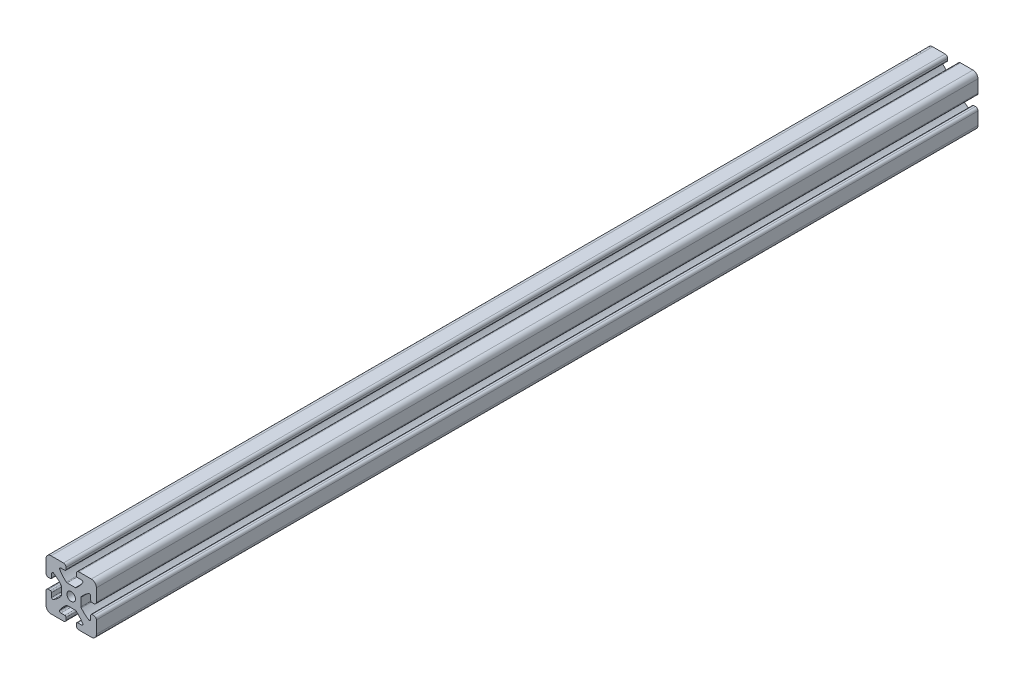
from build123d import *

# Parameters (mm, degrees)
SKETCH1_R           = 3.4
BOSS_EXTRUDE1_DEPTH = 700


with BuildPart() as part:
    # Sketch1 → Boss-Extrude1 (new body)
    with BuildSketch(Plane.XY):
        with BuildLine():
            Line((-72.552625451, -20.1458069), (-75.708839475, -20.1458069))
            ThreePointArc((-75.708839475, -20.1458069), (-76.585125865, -19.62759748), (-76.55321253, -18.610051226))
            ThreePointArc((-76.55321253, -18.610051226), (-74.186362214, -15.403020453), (-71.332517782, -12.620467892))
            ThreePointArc((-71.332517782, -12.620467892), (-71.036129936, -12.453644757), (-70.700972516, -12.3958069))
            Line((-70.700972516, -12.3958069), (-67.452625451, -12.3958069))
            Line((-67.452625451, -12.3958069), (-64.204278386, -12.3958069))
            ThreePointArc((-64.204278386, -12.3958069), (-63.869120967, -12.453644757), (-63.572733121, -12.620467892))
            ThreePointArc((-63.572733121, -12.620467892), (-60.718888688, -15.403020453), (-58.352038372, -18.610051226))
            ThreePointArc((-58.352038372, -18.610051226), (-58.320125037, -19.62759748), (-59.196411427, -20.1458069))
            Line((-59.196411427, -20.1458069), (-62.352625451, -20.1458069))
            ThreePointArc((-62.352625451, -20.1458069), (-63.059732232, -20.438700119), (-63.352625451, -21.1458069))
            Line((-63.352625451, -21.1458069), (-63.352625451, -22.6458069))
            ThreePointArc((-63.352625451, -22.6458069), (-62.766839013, -24.060020463), (-61.352625451, -24.6458069))
            Line((-61.352625451, -24.6458069), (-51.452625451, -24.6458069))
            ThreePointArc((-51.452625451, -24.6458069), (-48.624198326, -23.474234025), (-47.452625451, -20.6458069))
            Line((-47.452625451, -20.6458069), (-47.452625451, -10.7458069))
            ThreePointArc((-47.452625451, -10.7458069), (-48.038411889, -9.331593338), (-49.452625451, -8.7458069))
            Line((-49.452625451, -8.7458069), (-50.952625451, -8.7458069))
            ThreePointArc((-50.952625451, -8.7458069), (-51.659732232, -9.038700119), (-51.952625451, -9.7458069))
            Line((-51.952625451, -9.7458069), (-51.952625451, -12.902020924))
            ThreePointArc((-51.952625451, -12.902020924), (-52.470834871, -13.778307314), (-53.488381126, -13.74639398))
            ThreePointArc((-53.488381126, -13.74639398), (-56.695411898, -11.379543663), (-59.477964459, -8.525699231))
            ThreePointArc((-59.477964459, -8.525699231), (-59.644787594, -8.229311385), (-59.702625451, -7.894153965))
            Line((-59.702625451, -7.894153965), (-59.702625451, -4.6458069))
            Line((-59.702625451, -4.6458069), (-59.702625451, -1.397459836))
            ThreePointArc((-59.702625451, -1.397459836), (-59.644787594, -1.062302416), (-59.477964459, -0.76591457))
            ThreePointArc((-59.477964459, -0.76591457), (-56.695411898, 2.087929862), (-53.488381126, 4.454780179))
            ThreePointArc((-53.488381126, 4.454780179), (-52.470834871, 4.486693513), (-51.952625451, 3.610407123))
            Line((-51.952625451, 3.610407123), (-51.952625451, 0.4541931))
            ThreePointArc((-51.952625451, 0.4541931), (-51.659732232, -0.252913682), (-50.952625451, -0.5458069))
            Line((-50.952625451, -0.5458069), (-49.452625451, -0.5458069))
            ThreePointArc((-49.452625451, -0.5458069), (-48.038411889, 0.039979537), (-47.452625451, 1.4541931))
            Line((-47.452625451, 1.4541931), (-47.452625451, 11.3541931))
            ThreePointArc((-47.452625451, 11.3541931), (-48.624198326, 14.182620224), (-51.452625451, 15.3541931))
            Line((-51.452625451, 15.3541931), (-61.352625451, 15.3541931))
            ThreePointArc((-61.352625451, 15.3541931), (-62.766839013, 14.768406662), (-63.352625451, 13.3541931))
            Line((-63.352625451, 13.3541931), (-63.352625451, 11.8541931))
            ThreePointArc((-63.352625451, 11.8541931), (-63.059732232, 11.147086318), (-62.352625451, 10.8541931))
            Line((-62.352625451, 10.8541931), (-59.196411427, 10.8541931))
            ThreePointArc((-59.196411427, 10.8541931), (-58.320125037, 10.335983679), (-58.352038372, 9.318437425))
            ThreePointArc((-58.352038372, 9.318437425), (-60.718888688, 6.111406652), (-63.572733121, 3.328854091))
            ThreePointArc((-63.572733121, 3.328854091), (-63.869120967, 3.162030956), (-64.204278386, 3.1041931))
            Line((-64.204278386, 3.1041931), (-67.452625451, 3.1041931))
            Line((-67.452625451, 3.1041931), (-70.700972516, 3.1041931))
            ThreePointArc((-70.700972516, 3.1041931), (-71.036129936, 3.162030956), (-71.332517782, 3.328854091))
            ThreePointArc((-71.332517782, 3.328854091), (-74.186362214, 6.111406652), (-76.55321253, 9.318437425))
            ThreePointArc((-76.55321253, 9.318437425), (-76.585125865, 10.335983679), (-75.708839475, 10.8541931))
            Line((-75.708839475, 10.8541931), (-72.552625451, 10.8541931))
            ThreePointArc((-72.552625451, 10.8541931), (-71.84551867, 11.147086318), (-71.552625451, 11.8541931))
            Line((-71.552625451, 11.8541931), (-71.552625451, 13.3541931))
            ThreePointArc((-71.552625451, 13.3541931), (-72.138411889, 14.768406662), (-73.552625451, 15.3541931))
            Line((-73.552625451, 15.3541931), (-83.452625451, 15.3541931))
            ThreePointArc((-83.452625451, 15.3541931), (-86.281052576, 14.182620224), (-87.452625451, 11.3541931))
            Line((-87.452625451, 11.3541931), (-87.452625451, 1.4541931))
            ThreePointArc((-87.452625451, 1.4541931), (-86.866839013, 0.039979537), (-85.452625451, -0.5458069))
            Line((-85.452625451, -0.5458069), (-83.952625451, -0.5458069))
            ThreePointArc((-83.952625451, -0.5458069), (-83.24551867, -0.252913682), (-82.952625451, 0.4541931))
            Line((-82.952625451, 0.4541931), (-82.952625451, 3.610407123))
            ThreePointArc((-82.952625451, 3.610407123), (-82.434416031, 4.486693513), (-81.416869776, 4.454780179))
            ThreePointArc((-81.416869776, 4.454780179), (-78.209839004, 2.087929862), (-75.427286443, -0.76591457))
            ThreePointArc((-75.427286443, -0.76591457), (-75.260463308, -1.062302416), (-75.202625451, -1.397459836))
            Line((-75.202625451, -1.397459836), (-75.202625451, -4.6458069))
            Line((-75.202625451, -4.6458069), (-75.202625451, -7.894153965))
            ThreePointArc((-75.202625451, -7.894153965), (-75.260463308, -8.229311385), (-75.427286443, -8.525699231))
            ThreePointArc((-75.427286443, -8.525699231), (-78.209839004, -11.379543663), (-81.416869776, -13.74639398))
            ThreePointArc((-81.416869776, -13.74639398), (-82.434416031, -13.778307314), (-82.952625451, -12.902020924))
            Line((-82.952625451, -12.902020924), (-82.952625451, -9.7458069))
            ThreePointArc((-82.952625451, -9.7458069), (-83.24551867, -9.038700119), (-83.952625451, -8.7458069))
            Line((-83.952625451, -8.7458069), (-85.452625451, -8.7458069))
            ThreePointArc((-85.452625451, -8.7458069), (-86.866839013, -9.331593338), (-87.452625451, -10.7458069))
            Line((-87.452625451, -10.7458069), (-87.452625451, -20.6458069))
            ThreePointArc((-87.452625451, -20.6458069), (-86.281052576, -23.474234025), (-83.452625451, -24.6458069))
            Line((-83.452625451, -24.6458069), (-73.552625451, -24.6458069))
            ThreePointArc((-73.552625451, -24.6458069), (-72.138411889, -24.060020463), (-71.552625451, -22.6458069))
            Line((-71.552625451, -22.6458069), (-71.552625451, -21.1458069))
            ThreePointArc((-71.552625451, -21.1458069), (-71.84551867, -20.438700119), (-72.552625451, -20.1458069))
        make_face()
        with Locations((-67.452625451, -4.6458069)):
            Circle(SKETCH1_R, mode=Mode.SUBTRACT)
    extrude(amount=BOSS_EXTRUDE1_DEPTH)


solid = part.part
